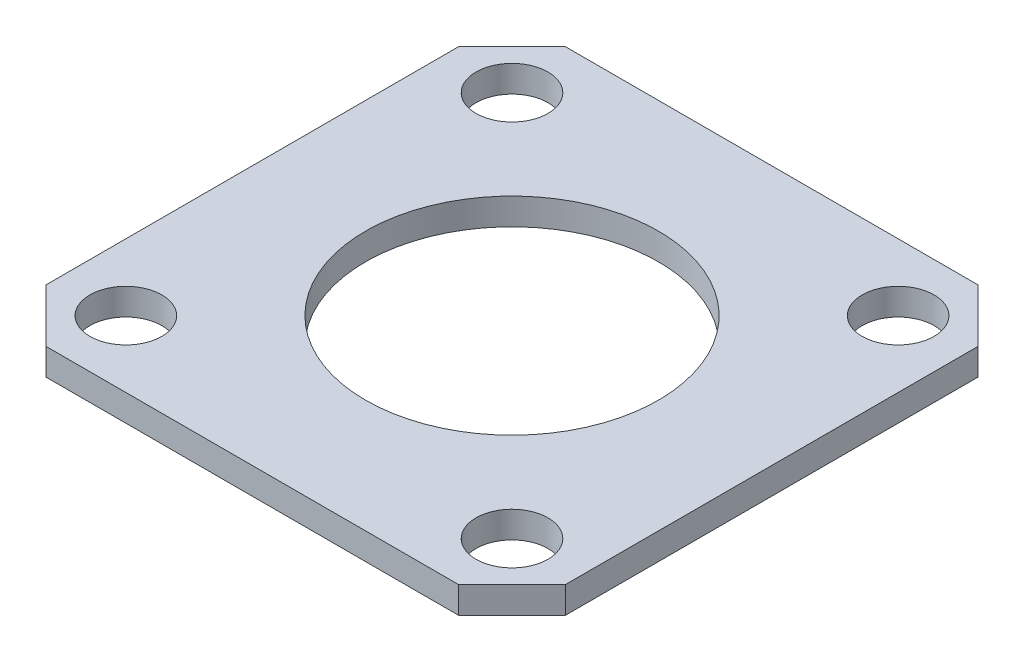
from build123d import *

# Parameters (mm, degrees)
SKETCH1_R           = 5.5
BOSS_EXTRUDE1_DEPTH = 1
SKETCH2_R           = 1.35
CUT_EXTRUDE1_DEPTH  = 1


with BuildPart() as part:
    # Sketch1 → Boss-Extrude1 (new body)
    with BuildSketch(Plane(origin=(0, 0, 0), x_dir=(1, 0, 0), z_dir=(0, 1, 0))):
        Polygon((7.75, -9.75), (9.75, -7.75), (9.75, 7.75), (7.75, 9.75), (-7.75, 9.75), (-9.75, 7.75), (-9.75, -7.75), (-7.75, -9.75), align=None)
        with Locations(Location((0, 0, 0), (0, 0, 270))):
            Circle(SKETCH1_R, mode=Mode.SUBTRACT)
    extrude(amount=BOSS_EXTRUDE1_DEPTH)

    # Sketch2 → Cut-Extrude1 (cut)
    with BuildSketch(Plane(origin=(0, 1, 0), x_dir=(1, 0, 0), z_dir=(0, 1, 0))):
        with Locations(Location((-7.25, 7.25, 0), (0, 0, 270))):
            Circle(SKETCH2_R)
        with Locations(Location((7.25, 7.25, 0), (0, 0, 270))):
            Circle(SKETCH2_R)
        with Locations(Location((7.25, -7.25, 0), (0, 0, 270))):
            Circle(SKETCH2_R)
        with Locations(Location((-7.25, -7.25, 0), (0, 0, 270))):
            Circle(SKETCH2_R)
    extrude(amount=-CUT_EXTRUDE1_DEPTH, mode=Mode.SUBTRACT)


solid = part.part
